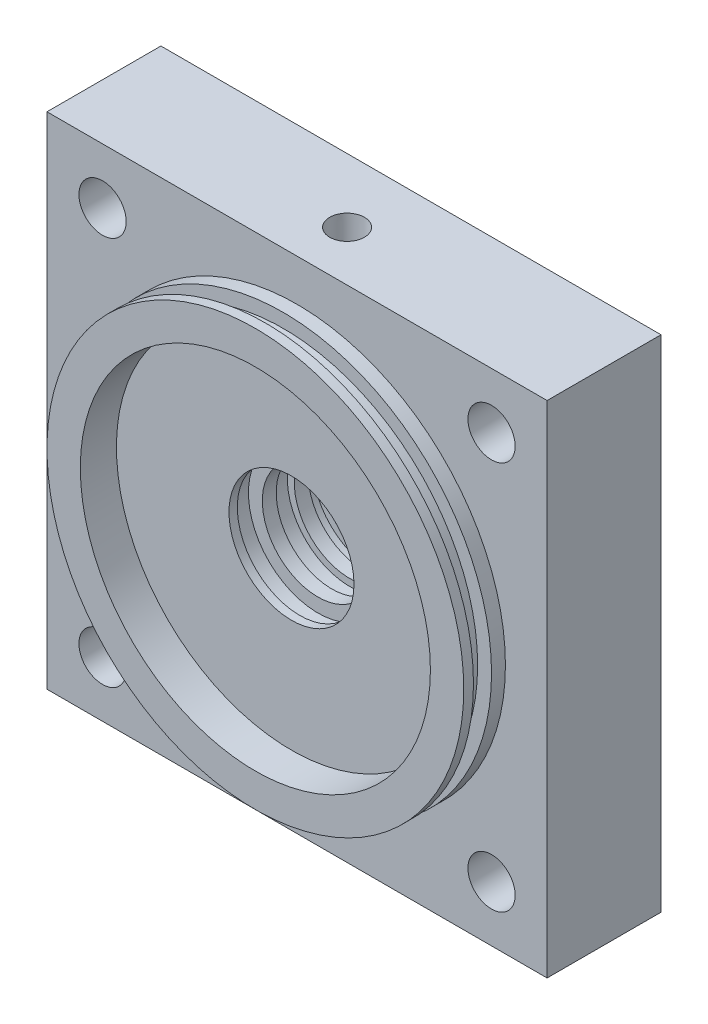
from build123d import *

# Parameters (mm, degrees)
SKETCH_1_W               = 180
SKETCH_1_H               = 180
EXTRUDE_1_DEPTH          = 41
SKETCH_2_R               = 75
EXTRUDE_2_DEPTH          = 15
SKETCH_3_R               = 63
CUT_EXTRUDE_1_DEPTH      = 13
SKETCH_4_W               = 6.5
SKETCH_4_H               = 5
CUT_EXTRUDE_2_REACH      = 136.347
CUT_EXTRUDE_2_END_RADIUS = 5.5626
SKETCH_9_R               = 3
CUT_EXTRUDE_3_REACH      = 141.054
SKETCH_10_R              = 8.5


with BuildPart() as part:
    # 草图1 → 凸台-拉伸1 (new body)
    with BuildSketch(Plane.XY):
        Rectangle(SKETCH_1_W, SKETCH_1_H)
    extrude(amount=EXTRUDE_1_DEPTH)

    # 草图2 → 凸台-拉伸2 (add)
    with BuildSketch(Plane.XY.offset(41)):
        Circle(SKETCH_2_R)
    extrude(amount=EXTRUDE_2_DEPTH)

    # 草图3 → 切除-拉伸1 (cut)
    with BuildSketch(Plane.XY.offset(56)):
        Circle(SKETCH_3_R)
    extrude(amount=-CUT_EXTRUDE_1_DEPTH, mode=Mode.SUBTRACT)

    # 草图4 → 切除-旋转1 (revolve, cut)
    with BuildSketch(Plane(origin=(0, 0, 0), x_dir=(0, 0, -1), z_dir=(1, 0, 0)), mode=Mode.PRIVATE) as cut_revolve_1_sk:
        with Locations((-49.25, 72.5)):
            Rectangle(SKETCH_4_W, SKETCH_4_H)
    revolve(cut_revolve_1_sk.sketch.rotate(Axis((0, 0, 56), (0, 0, -1)), 90), axis=Axis((0, 0, 56), (0, 0, -1)), mode=Mode.SUBTRACT)

    # 草图6 → 1/4 NPT 螺纹孔1 (revolve, cut)
    with BuildSketch(Plane(origin=(0, 90, 23), x_dir=(0, 0, 1), z_dir=(1, 0, 0))):
        Polygon((0, 0), (0, 36.342347279), (5.5626, 33), (5.5626, 10.02), (5.943676082, 10.02), (6.2436883, 0), align=None)
    revolve(axis=Axis((0, 96.35, 23), (0, -1, 0)), mode=Mode.SUBTRACT)

    # 草图8 → 切除-旋转2 (revolve, cut)
    with BuildSketch(Plane(origin=(0, 0, 0), x_dir=(1, 0, 0), z_dir=(0, 1, 0))):
        Polygon((0, -56), (22.5, -56), (22.5, -40), (25, -40), (25, -33.5), (20, -33.5), (20, -28.5), (22.5, -28.5), (22.5, -22), (20, -22), (20, -17), (22.5, -17), (22.5, -13), (20, -13), (20, -8), (22.5, -8), (22.5, -4), (20, -4), (20, 0), (0, 0), align=None)
    revolve(axis=Axis((0, 0, 56), (0, 0, -1)), mode=Mode.SUBTRACT)

    # 切除-拉伸2: up to this cylinder (the profile starts outside it)
    cut_extrude_2_end = Plane(origin=(0, 60, 23), z_dir=(0, 1, 0)) * Cylinder(CUT_EXTRUDE_2_END_RADIUS, 284.8192, mode=Mode.PRIVATE)
    # 草图9 → 切除-拉伸2 (cut, up to the surface)
    with BuildSketch(Plane.XY.offset(43), mode=Mode.PRIVATE) as cut_extrude_2_sk1:
        with Locations(Location((0, 60, 0), (0, 0, 270))):
            Circle(SKETCH_9_R)
    cut_extrude_2_tool1 = extrude(cut_extrude_2_sk1.sketch, amount=-CUT_EXTRUDE_2_REACH, mode=Mode.PRIVATE) - cut_extrude_2_end
    add(cut_extrude_2_tool1.solids().sort_by_distance((0, 60, 43))[0], mode=Mode.SUBTRACT)

    # 草图10 → 切除-拉伸3 (cut, up to next)
    with BuildSketch(Plane(origin=(0, 0, 0), x_dir=(-1, 0, 0), z_dir=(0, 0, -1)), mode=Mode.PRIVATE) as cut_extrude_3_sk1:
        with Locations((-70, 70)):
            Circle(SKETCH_10_R)
    cut_extrude_3_tool1 = extrude(cut_extrude_3_sk1.sketch, amount=-CUT_EXTRUDE_3_REACH, mode=Mode.PRIVATE) & part.part
    # 草图10 → 切除-拉伸3 (cut, up to next)
    with BuildSketch(Plane(origin=(0, 0, 0), x_dir=(-1, 0, 0), z_dir=(0, 0, -1)), mode=Mode.PRIVATE) as cut_extrude_3_sk2:
        with Locations((70, 70)):
            Circle(SKETCH_10_R)
    cut_extrude_3_tool2 = extrude(cut_extrude_3_sk2.sketch, amount=-CUT_EXTRUDE_3_REACH, mode=Mode.PRIVATE) & part.part
    # 草图10 → 切除-拉伸3 (cut, up to next)
    with BuildSketch(Plane(origin=(0, 0, 0), x_dir=(-1, 0, 0), z_dir=(0, 0, -1)), mode=Mode.PRIVATE) as cut_extrude_3_sk3:
        with Locations((70, -70)):
            Circle(SKETCH_10_R)
    cut_extrude_3_tool3 = extrude(cut_extrude_3_sk3.sketch, amount=-CUT_EXTRUDE_3_REACH, mode=Mode.PRIVATE) & part.part
    # 草图10 → 切除-拉伸3 (cut, up to next)
    with BuildSketch(Plane(origin=(0, 0, 0), x_dir=(-1, 0, 0), z_dir=(0, 0, -1)), mode=Mode.PRIVATE) as cut_extrude_3_sk4:
        with Locations((-70, -70)):
            Circle(SKETCH_10_R)
    cut_extrude_3_tool4 = extrude(cut_extrude_3_sk4.sketch, amount=-CUT_EXTRUDE_3_REACH, mode=Mode.PRIVATE) & part.part
    add(cut_extrude_3_tool1.solids().sort_by_distance((70, 70, 0))[0], mode=Mode.SUBTRACT)
    add(cut_extrude_3_tool2.solids().sort_by_distance((-70, 70, 0))[0], mode=Mode.SUBTRACT)
    add(cut_extrude_3_tool3.solids().sort_by_distance((-70, -70, 0))[0], mode=Mode.SUBTRACT)
    add(cut_extrude_3_tool4.solids().sort_by_distance((70, -70, 0))[0], mode=Mode.SUBTRACT)


solid = part.part
